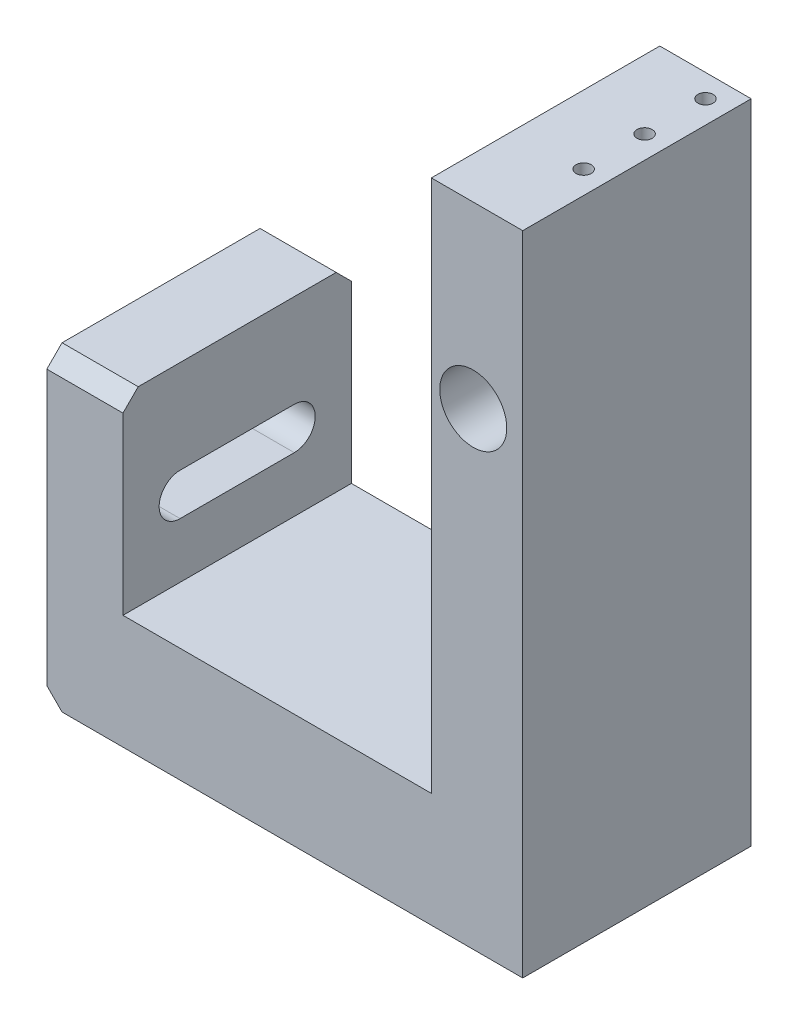
SolidWorks part; units mm, degrees
ref_plane "Front Plane" through (0, 0, 0) normal (0, 0, 1) x (1, 0, 0)
ref_plane "Top Plane" through (0, 0, 0) normal (0, 1, 0) x (1, 0, 0)
ref_plane "Right Plane" through (0, 0, 0) normal (1, 0, 0) x (0, 0, -1)
sketch "Sketch1" plane through (0, 0, 0) normal (0, 0, 1) x (1, 0, 0)
  line L0 (-10, 40) -> (-10, 0)
  line L1 (-10, 40) -> (0, 40)
  line L2 (0, 40) -> (0, 15)
  line L3 (0, 15) -> (40.5, 15)
  line L4 (40.5, 15) -> (40.5, 85)
  line L6 (40.5, 85) -> (52.5, 85)
  line L7 (52.5, 85) -> (52.5, 0)
  line L8 (52.5, 0) -> (-10, 0)
  line L9 (0, 0) -> (-58.3826, 0) construction
  dimension "D1" = 40.5
  dimension "D2" = 10
  dimension "D4" = 12
  dimension "D5" = 85
  dimension "D6" = 15
  dimension "D7" = 40
extrude "Boss-Extrude1" add sketch "Sketch1" along normal blind 30
sketch "Sketch2" plane through (0, 85, 0) normal (0, 1, 0) x (1, 0, 0)
  line L2 (52.5, -15) -> (35.0033, -15) construction
  line L3 (52.5, -30) -> (52.5, 0) construction
  circle A0 centre (49.5, -3) radius 1
  circle A1 centre (49.5, -11) radius 1
  circle A2 centre (49.5, -19) radius 1
  circle A4 centre (49.5, -27) radius 1 [skipped]
  dimension "D1" = 2
  dimension "D2" = 12
  dimension "D4" = 3
  dimension "D3" = 4
extrude "Cut-Extrude1" cut sketch "Sketch2" against normal blind 25
sketch "Sketch3" plane through (0, 0, 30) normal (0, 0, 1) x (1, 0, 0)
  line L0 (46, 61.5) -> (49.4561, 61.5) construction
  line L2 (52.5, 0) -> (52.5, 85) construction
  line L3 (-10, 0) -> (52.5, 0) construction
  circle A0 centre (46, 61.5) radius 3
  dimension "D1" = 6
  dimension "D2" = 6.5
  dimension "D3" = 61.5
extrude "Cut-Extrude2" cut sketch "Sketch3" against normal blind 28
sketch "Sketch4" plane through (0, 0, 0) normal (0, -1, 0) x (1, 0, 0)
  line L0 (52.5, 15) -> (26.4467, 15) construction
  line L1 (52.5, 30) -> (52.5, 0) construction
  circle A0 centre (46, 15) radius 3
  dimension "D1" = 6.5
  dimension "D2" = 6
extrude "Cut-Extrude3" cut sketch "Sketch4" against normal blind 61.5
sketch "Sketch5" plane through (-10, 0, 0) normal (-1, 0, 0) x (0, 0, 1)
  line L0 (7.5, 25) -> (22.5, 25) construction
  line L1 (7.5, 27.75) -> (22.5, 27.75)
  line L2 (7.5, 22.25) -> (22.5, 22.25)
  line L3 (15, 0) -> (15, 10.6719) construction
  line L4 (30, 0) -> (0, 0) construction
  arc A0 (7.5, 27.75) -> (7.5, 22.25) centre (7.5, 25) ccw
  arc A1 (22.5, 22.25) -> (22.5, 27.75) centre (22.5, 25) ccw
  point P2 (15, 25)
  dimension "D1" = 5.5
  dimension "D2" = 15
  dimension "D3" = 25
extrude "Cut-Extrude4" cut sketch "Sketch5" against normal blind 20
chamfer "Chamfer1" distance 2 angle 45 3 edges at (-10, 0, 15) (-5, 40, 30) (-5, 40, 0)
hole_wizard "G1/8 Tapped Hole1" positions "Sketch9" profile "Sketch8" tap size "G1/8" standard "Iso"
sketch "Sketch9" plane through (0, 0, 0) normal (0, -1, 0) x (1, 0, 0)
  point P0 (46, 15)
sketch "Sketch8" plane through (46, 0, 15) normal (1, 0, 0) x (0, 0, -1)
  line L0 (0, 0) -> (0, 15.3638)
  line L1 (0, 15.3638) -> (4.4, 12.72)
  line L2 (4.4, 12.72) -> (4.4, 0)
  line L5 (4.4, 0) -> (0, 0)
  line L10 (0, 15.3638) -> (-4.4, 12.72) construction
  line L11 (0, -6.35) -> (0, 107.95) construction
  dimension "螺纹孔钻头直径" = 8.8
  dimension "螺纹孔钻头深度" = 12.72
  dimension "导头角度" = 118
cosmetic thread "Cosmetic Thread3" parameters "D1"=10, "D2"=9.728
hole_wizard "G1/8 Tapped Hole2" positions "Sketch11" profile "Sketch10" tap size "G1/8" standard "Gb"
sketch "Sketch11" plane through (0, 0, 30) normal (0, 0, 1) x (1, 0, 0)
  point P0 (46, 61.5)
sketch "Sketch10" plane through (46, 61.5, 30) normal (1, 0, 0) x (0, -1, 0)
  line L0 (0, 0) -> (0, 13.3638)
  line L1 (0, 13.3638) -> (4.4, 10.72)
  line L2 (4.4, 10.72) -> (4.4, 0)
  line L5 (4.4, 0) -> (0, 0)
  line L10 (0, 13.3638) -> (-4.4, 10.72) construction
  line L11 (0, -6.35) -> (0, 107.95) construction
  dimension "螺纹孔钻头直径" = 8.8
  dimension "螺纹孔钻头深度" = 10.72
  dimension "导头角度" = 118
cosmetic thread "Cosmetic Thread4" parameters "D1"=8, "D2"=9.728
